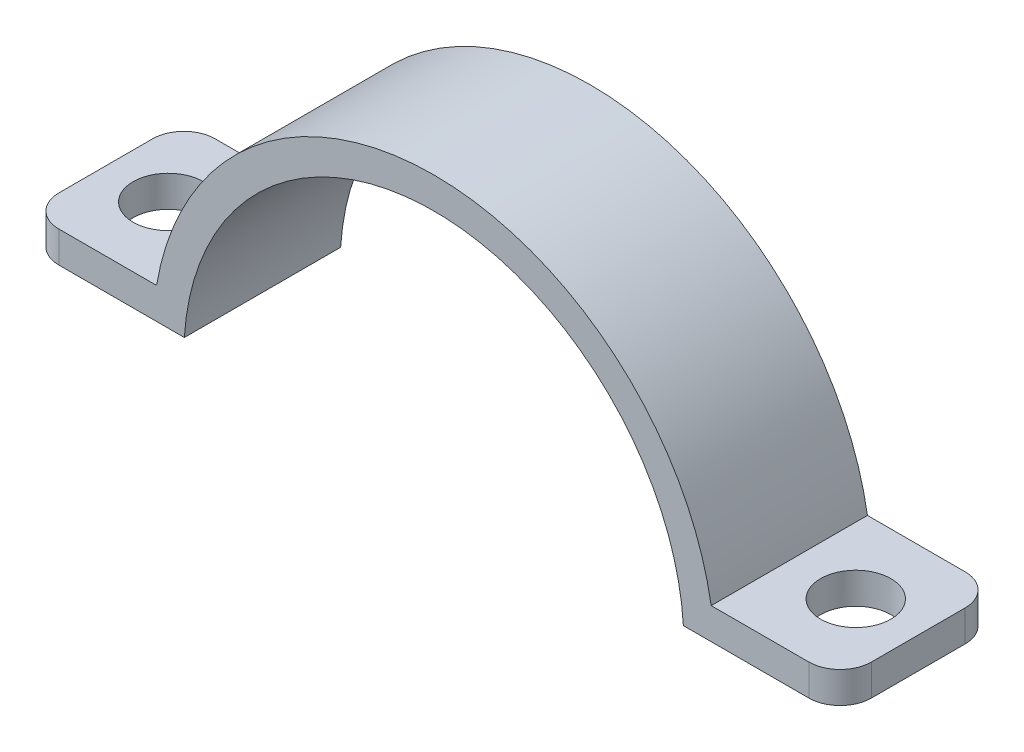
from build123d import *

# Parameters (mm, degrees)
EXTRUDE_THIN1_DEPTH      = 10
M4_CLEARANCE_HOLE1_D     = 4.5
M4_CLEARANCE_HOLE1_DEPTH = 124.5
M4_CLEARANCE_HOLE1_TIP   = 1.351936393
FILLET1_R                = 2


with BuildPart() as part:
    # Sketch1 → Extrude-Thin1 (new body)
    with BuildSketch(Plane.XY):
        with BuildLine():
            Line((41.968719423, 0), (31.937438845, 0))
            ThreePointArc((31.937438845, 0), (15.968719423, 15), (0, 0))
            Line((0, 0), (-10.031280577, 0))
            Line((-10.031280577, 0), (-10.031280577, 2))
            Line((-10.031280577, 2), (-1.779519927, 2))
            ThreePointArc((-1.779519927, 2), (15.968719423, 17), (33.716958772, 2))
            Line((33.716958772, 2), (41.968719423, 2))
            Line((41.968719423, 2), (41.968719423, 0))
        make_face()
    extrude(amount=-EXTRUDE_THIN1_DEPTH)

    # M4 Clearance Hole1
    with Locations(Plane(origin=(0, 2, 0), x_dir=(1, 0, 0), z_dir=(0, 1, 0))):
        with Locations((-6.031280577, 5), (37.968719423, 5)):
            Hole(M4_CLEARANCE_HOLE1_D / 2, depth=M4_CLEARANCE_HOLE1_DEPTH)
            with Locations((0, 0, -(M4_CLEARANCE_HOLE1_DEPTH + M4_CLEARANCE_HOLE1_TIP / 2))):  # 118° drill point
                Cone(0, M4_CLEARANCE_HOLE1_D / 2, M4_CLEARANCE_HOLE1_TIP, mode=Mode.SUBTRACT)

    # Fillet1
    fillet1_edges = [part.edges().sort_by_distance(p)[0] for p in [
        (-10.031280577, 1, -10),
        (41.968719423, 1, -10),
        (-10.031280577, 1, 0),
        (41.968719423, 1, 0),
    ]]
    fillet(fillet1_edges, radius=FILLET1_R)


solid = part.part
